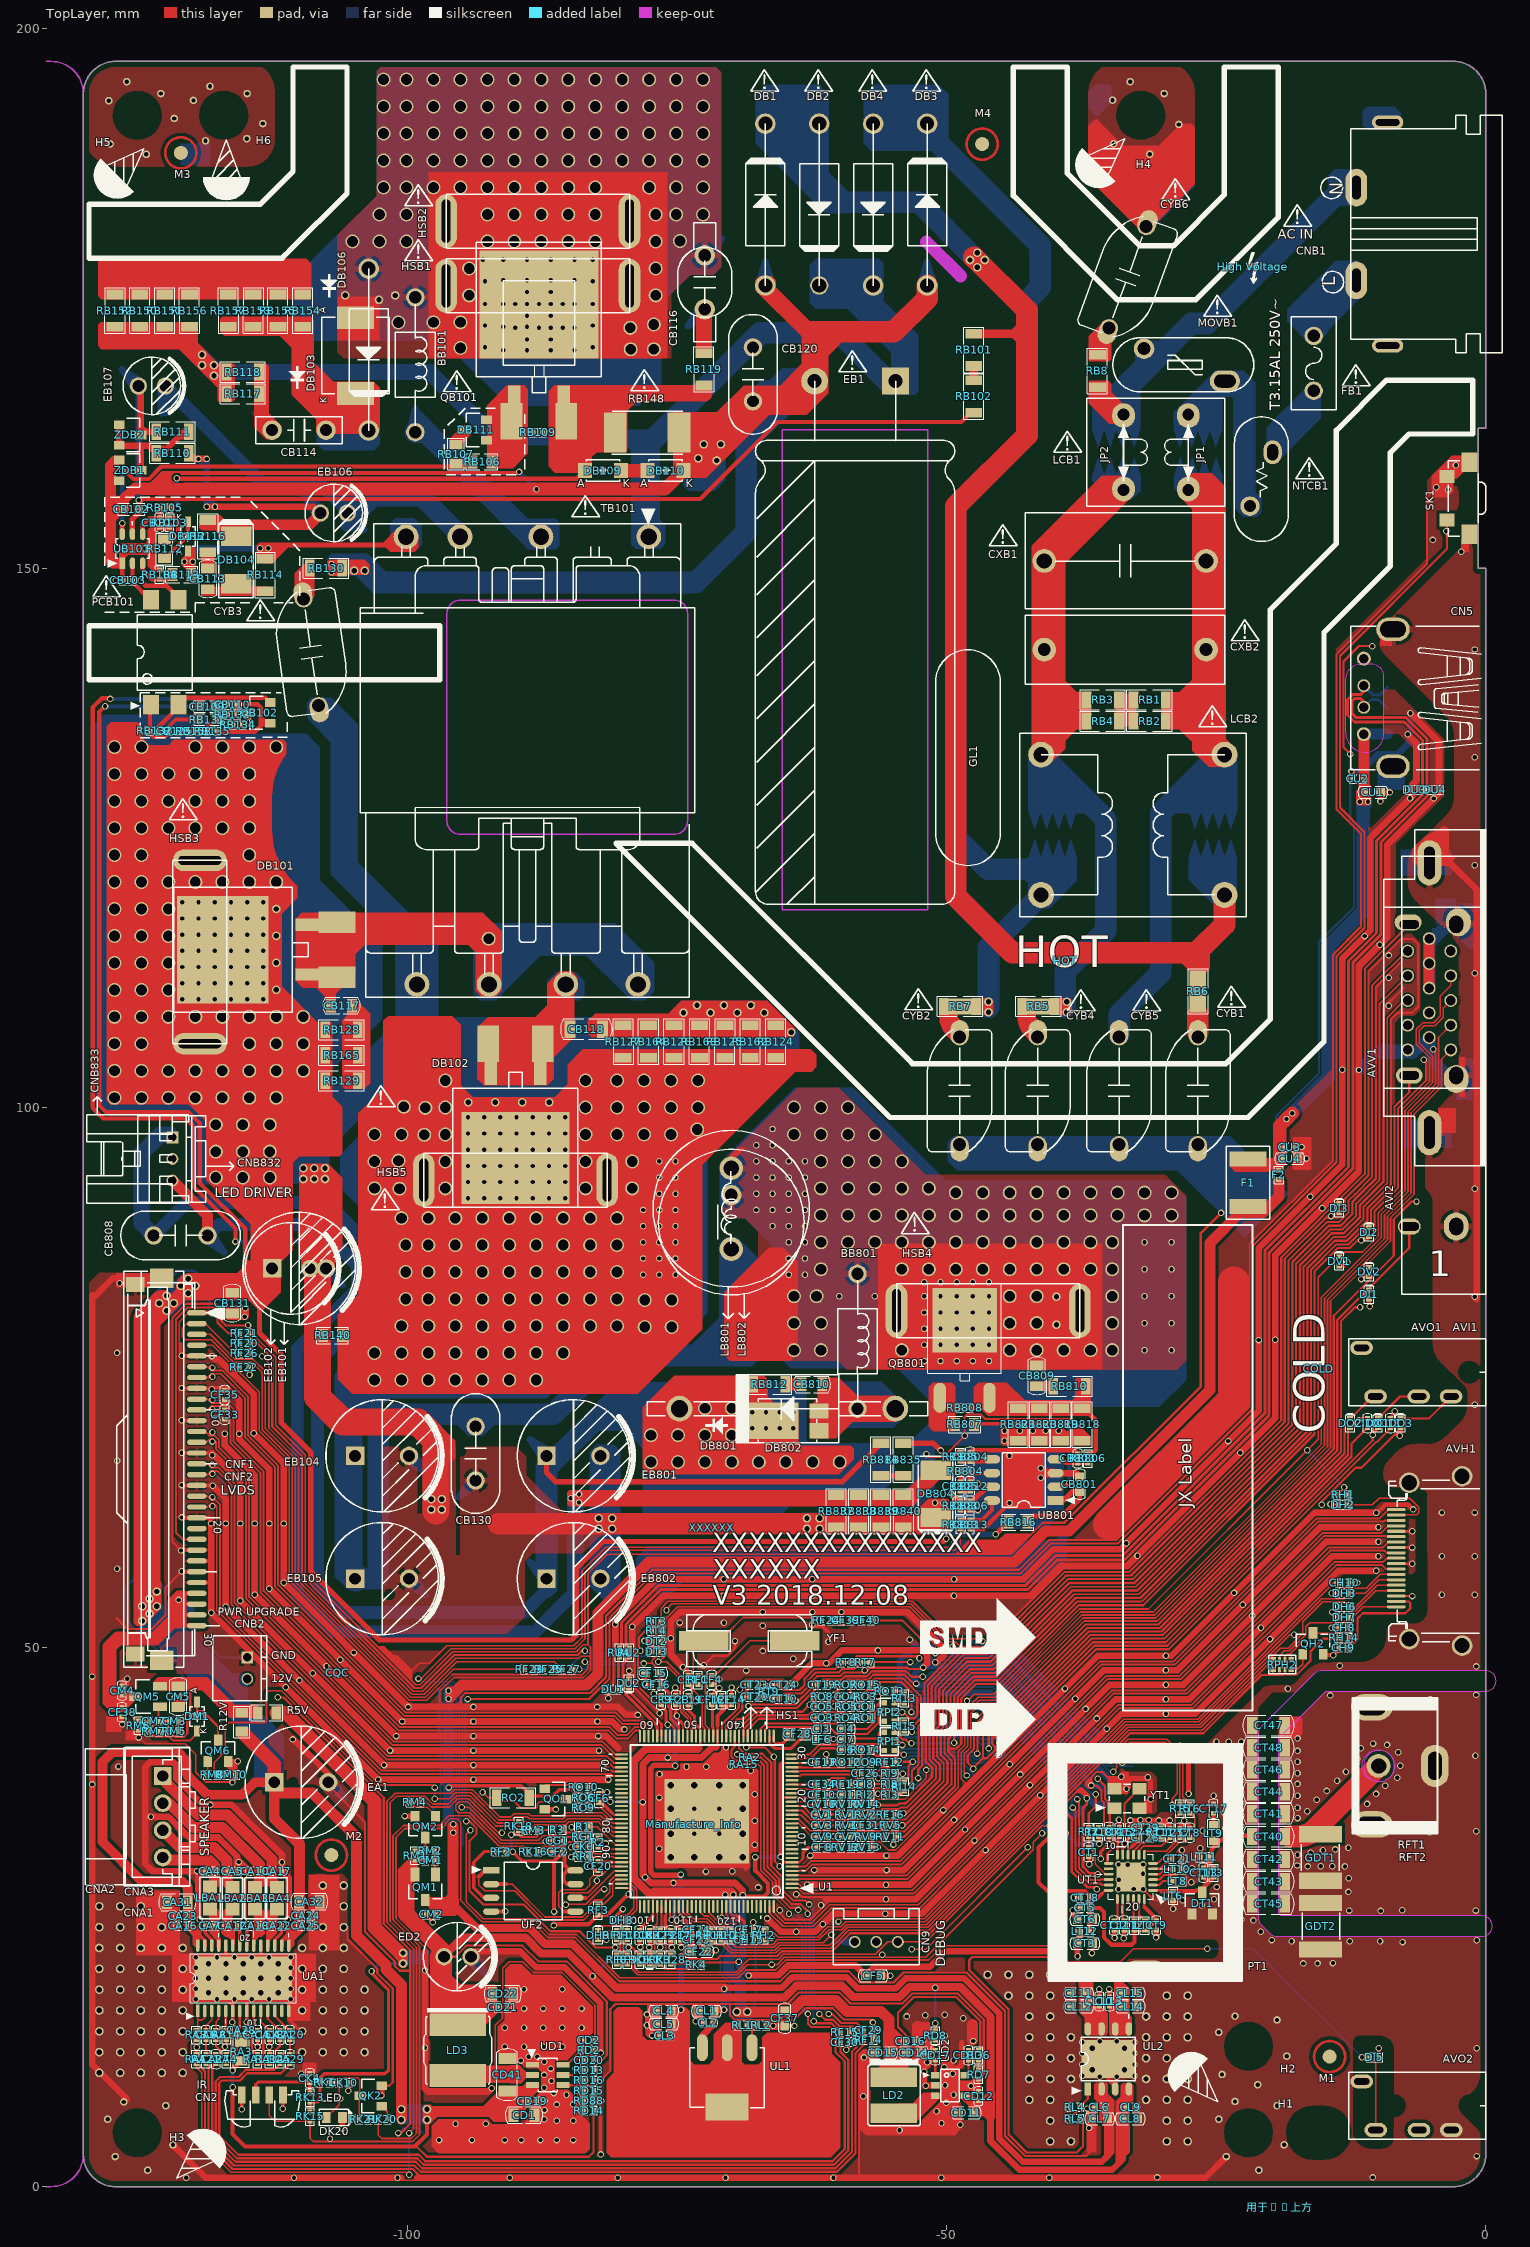
[diagram p0: TopLayer view]
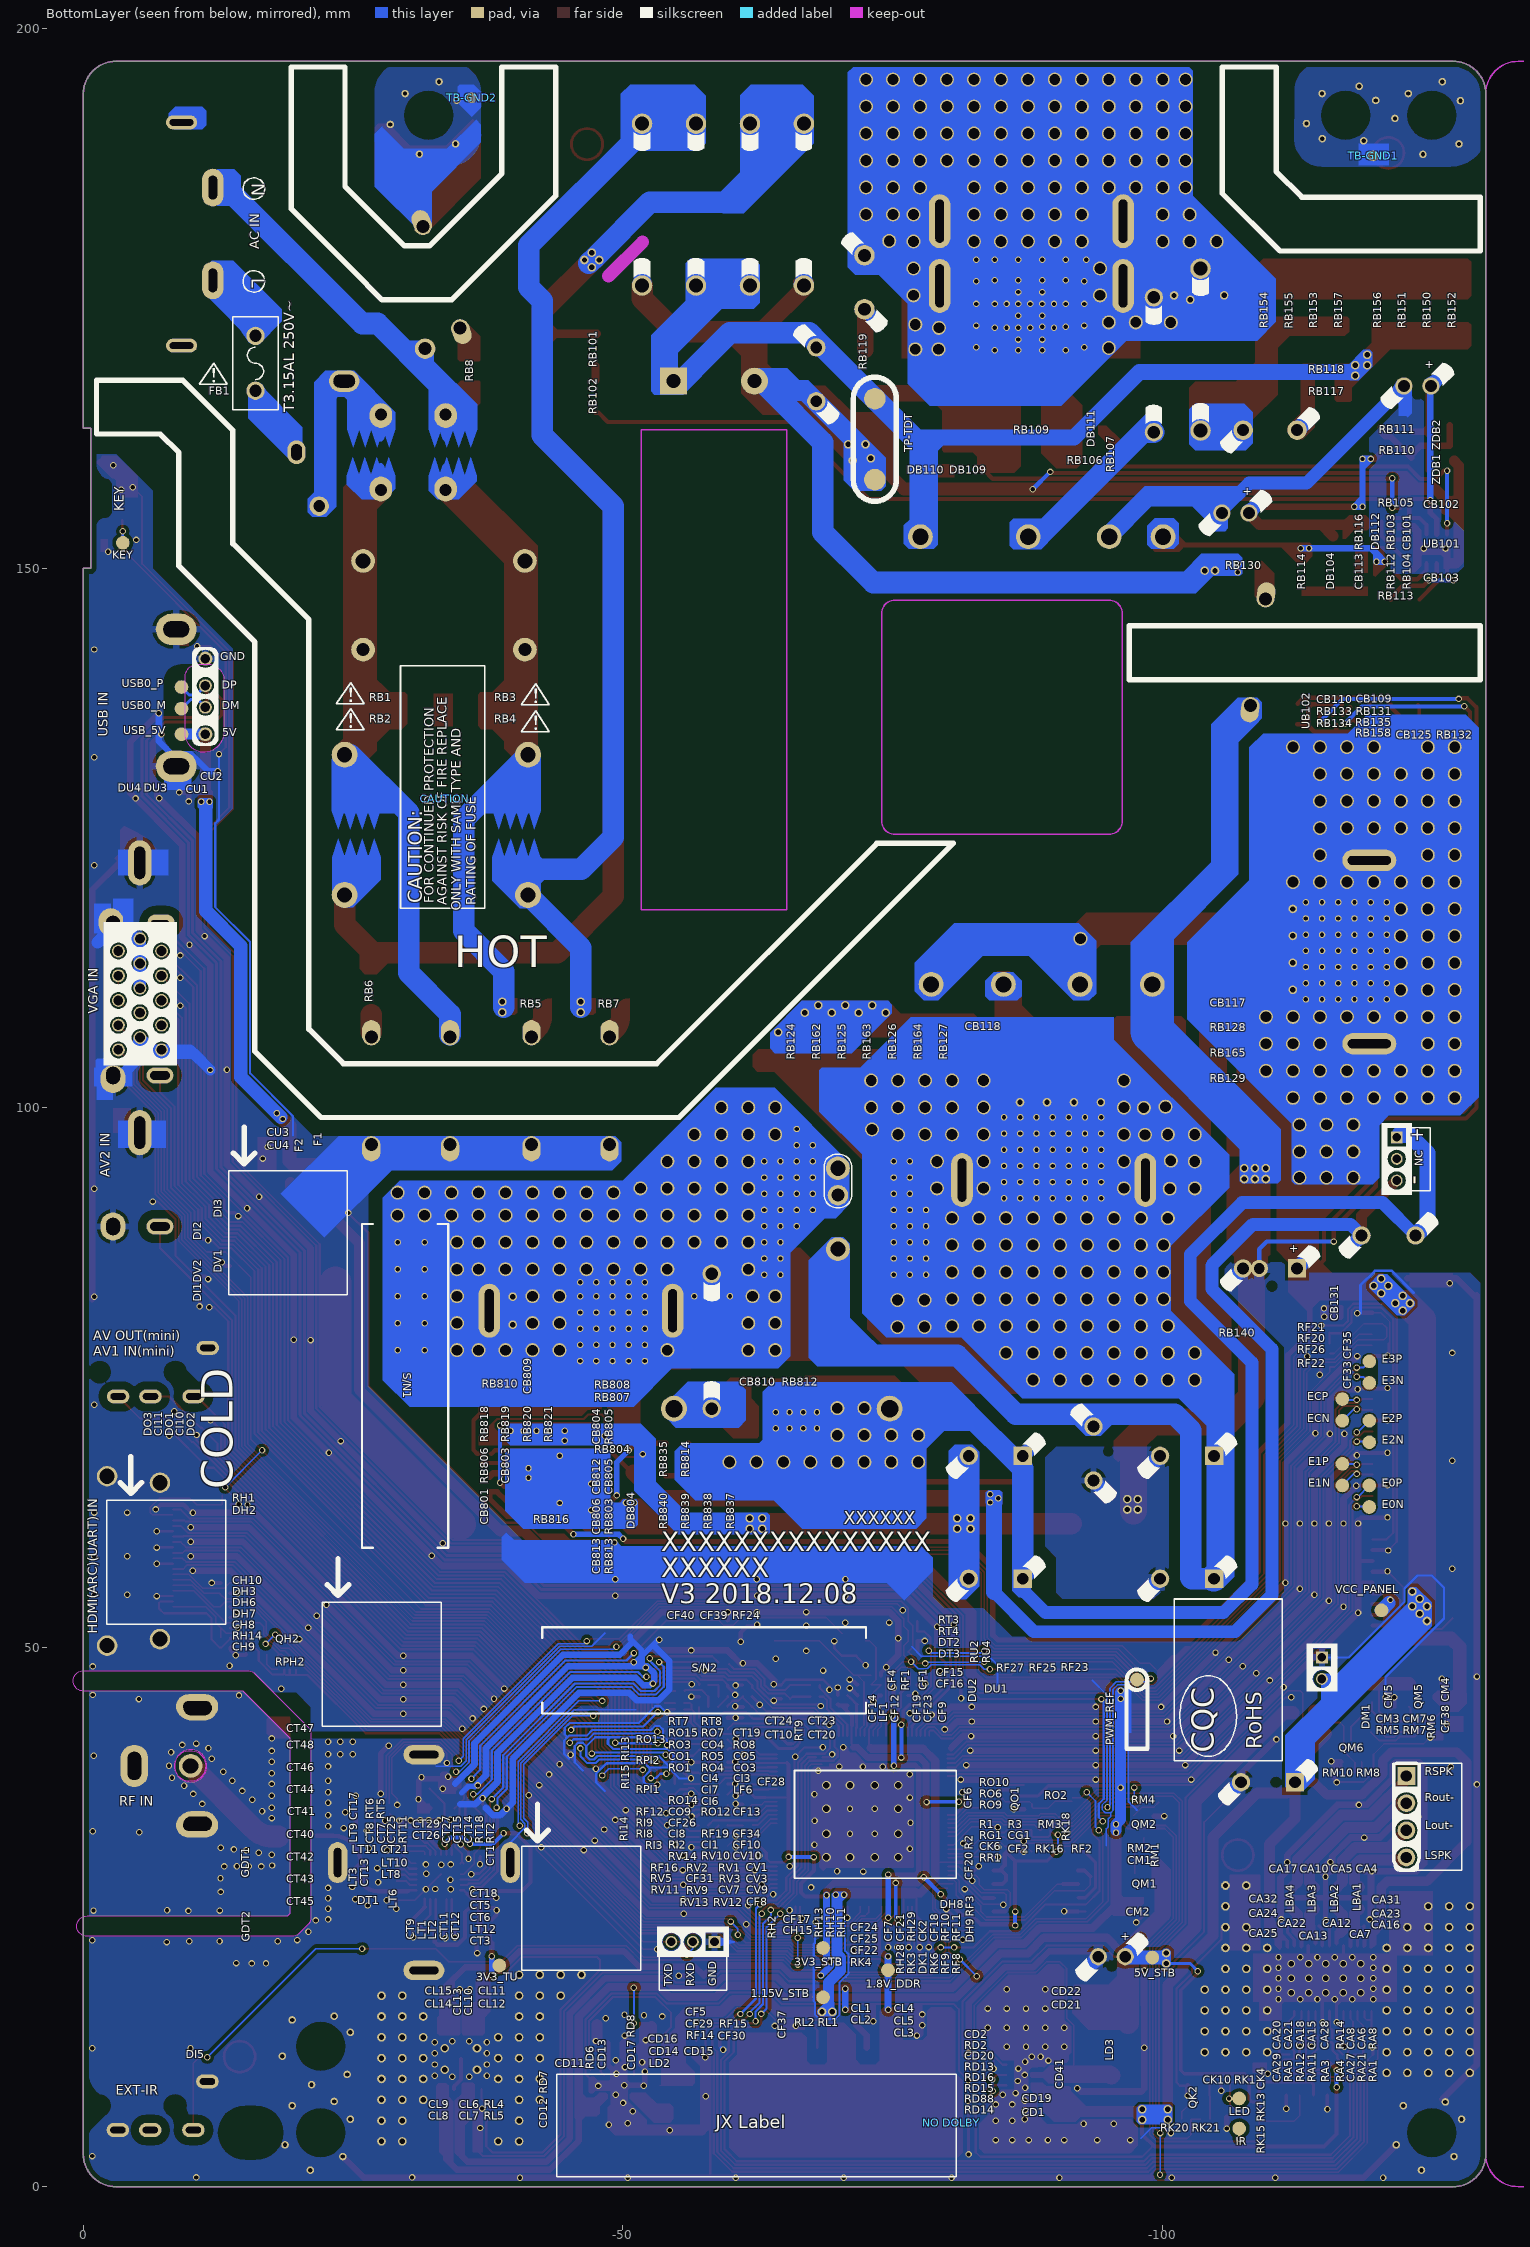
[diagram p1: BottomLayer view, seen from below]
# Altium PCB MISC84438.PcbDoc (part 1 of 15)
Units mm, origin at the board's own origin, x right, y up, seen from the top; angles counter-clockwise.
Board outline 130 x 197 mm, 2 copper layers (TopLayer, BottomLayer), stack 1.571 mm thick; 574 components, 314 nets, 2636 pads, 811 vias.

## Layer stack, top to bottom
TopLayer: signal copper 0.0356
Dielectric: core 1.5, FR-4, Dk 4.8
BottomLayer: signal copper 0.0356

## Board outline
-130,3 ccw(c-127,3) -127,0 -3,0 ccw(c-3,3) 0,3 0,150 -0.703,150 -0.703,163 0,163 0,194 ccw(c-3,194) -3,197 -127,197 ccw(c-127,194) -130,194

## Design rules (kind name [scope] priority, off if disabled: settings)
Clearance ■KEEPOUT_18mil [(IsTrack Or IsArc) And (AsMM(Width) < 1) And IsKeepOut vs Not IsPad] p1: gap=0.457
Clearance ■HOT_7.2mm [InNetClass('HOT') vs InNetClass('All Nets') And (Not InNetClass('HOT'))] p2: gap=7.2
Clearance ■DFM_NPTH_10mil [(IsPadHoleValid And (PadIsPlated=false) Or IsPad And ((AsMM(PadXSize_AllLayers) < 1) or (AsMM(PadYSize_AllLayers) < 1 )) And IsKeepout) OR HasFootprintPad('ASSE*','0') vs Not IsPad] p3: gap=0.254
Clearance ■DFM_20mil [(IsTrack or IsArc or IsPad) And IsKeepOut vs IsTrack or IsArc or InPoly] p4: gap=0.508
Clearance ■PWR_A12_8mil [(InNetClass('PWR_A12_8mil') or InNet('*12V*') or InNet('*24V*') or InNet('*PVCC*') or InNet('*19V*') or InNet('*AMP*POWER*') or InNet('*AMP*VCC*') or InNet('*LNB*')) and Not IsPad vs Not InPoly] p5: gap=0.203
Clearance ■PS_L2All_3.2mm [InNet('L-1') vs InNet('*')] p6: gap=3.2
Clearance ■PS_L2LN_1.5mm [InNet('L') Or InNet('L-2') Or InNet('L-3') Or InNet('L-4') Or InNet('L-5') Or InNet('L-6') vs InNet('L-N') And Not(InNet('L') Or InNet('L-2') Or InNet('L-3') Or InNet('L-4') Or InNet('L-5') Or InNet('L-6'))] p7: gap=1.5
Clearance ■PS_N2LN_1.5mm [InNet('N') OR InNet('N-1') OR InNet('N-2') OR InNet('N-3') OR InNet('N-4') OR InNet('N-5') OR InNet('N-6') vs InNet('L-N') And Not (InNet('N') OR InNet('N-1') OR InNet('N-2') OR InNet('N-3') OR InNet('N-4') OR InNet('N-5') OR InNet('N-6'))] p8: gap=1.5
Clearance ■PS_L2LN_3mm [InNet('L') Or InNet('L-2') Or InNet('L-3') Or InNet('L-4') Or InNet('L-5') Or InNet('L-6') vs InNet('*') And Not (InNet('L-N') Or InNet('L') Or InNet('L-2') Or InNet('L-3') Or InNet('L-4') Or InNet('L-5') Or InNet('L-6') Or OnLayer('KeepOutLayer'))] p9: gap=3
Clearance ■PS_N2LN_3mm [InNet('N') OR InNet('N-1') OR InNet('N-2') OR InNet('N-3') OR InNet('N-4') OR InNet('N-5') OR InNet('N-6') vs InNet('*') And Not (InNet('L-N') Or InNet('N') OR InNet('N-1') OR InNet('N-2') OR InNet('N-3') OR InNet('N-4') OR InNet('N-5') OR InNet('N-6') Or OnLayer('KeepOutLayer'))] p10: gap=3
Clearance ■SIP2GND_8mil [HasFootprint('SIP*') vs InPoly] p11: gap=0.203
Clearance ■Poly_4mil [InPolygonClass('Poly_4mil') vs Not InPoly] p12: gap=0.102
Clearance ■Poly_5mil [InPolygonClass('Poly_5mil') vs Not InPoly] p13: gap=0.127
Clearance ■Poly_6.2mil [InPolygonClass('Poly_6.2mil') vs Not InPoly] p14: gap=0.157
Clearance ■Poly_8mil [InPolygonClass('Poly_8mil') vs Not InPoly] p15: gap=0.203
Clearance ■ESD_10mil [HasFootprint('*IEC*') Or HasFootprint('*-F1*') Or HasFootprint('ANT-RF*')] p16: gap=0.254
Clearance ■ESD_20mil [HasFootprint('*SHIELD*')] p17: gap=0.508
Clearance ■C_RFGND_1.8mm [InNet('RFGND') vs Not (InNet('RF*IN*') OR InNet('NetCT28*'))] p18: gap=1.8
Clearance ■GND_12mil [InNet('GND') vs InPoly] p19: gap=0.305
Clearance ■ESD_30mil [(HasFootprint('SCART*') OR HasFootprint('AV*') OR HasFootprint('DB15*') OR HasFootprint('PHONE*')) vs OnBottomLayer] p20: gap=0.762
Clearance ■ESD_NT_30mil [HasFootprint('SCART*') Or HasFootprint('PHONE-HD-12') Or HasFootprint('PHONE-HD-17') Or HasFootprint('PHONE-HD-10') Or HasFootprint('PHONE-HD-26') vs InNet('GND') And OnTopLayer] p21: gap=0.762
Clearance ■DFM_TH_5mil [HasFootprint('GND') or HasFootprint('TP*') or HasFootprint('MARK*') or HasFootprint('SPARK_GAP') or HasFootprint('USB-HD-3-2') or HasFootprint('PHONE-HS-20') and Not IsRegion vs OnBottomlayer And IsPad OR IsPadHoleValid] p22: gap=0.127
Clearance ■DFM_HS60_5mil [InPadClass('HS60') vs InPadClass('HS60') OR IsPadHoleValid and not InPadClass('VIA5')] p23: gap=0.127
Clearance ■DFM_BCR_4mm [IsPadHoleValid vs IsBoardCutoutRegion] p24: gap=4
Clearance ■DFM_TH_4mm [OnBottomlayer And IsSMTPin vs IsPadHoleValid and not InPadClass('VIA5')] p25: gap=4
Clearance ■DFM_HS60_4mm [InPadClass('HS60') vs IsPad and OnBottomlayer] p26: gap=4
Clearance ■VIA2VIA_6.2mil [(IsVia OR InPadClass('VIA5')) And Not (IsVia And (AsMM(HoleDiameter) = 0.1)) vs (IsVia OR InPadClass('VIA5')) And Not (IsVia And (AsMM(HoleDiameter) = 0.1))] p27: gap=0.157
Clearance ■VIA2VIA_10.2mil [(IsVia OR InPadClass('VIA5')) And Not (IsVia And (AsMM(HoleDiameter) = 0.1)) vs (IsVia OR InPadClass('VIA5')) And Not (IsVia And (AsMM(HoleDiameter) = 0.1))] p28: gap=0.259
Clearance ■VIA2PAD_BGA_5mil [HasFootprint('BGA*') and IsPad vs (IsVia OR InPadClass('VIA5')) And Not (IsVia And (AsMM(HoleDiameter) = 0.1))] p29: gap=0.127
Clearance ■VIA2PAD_6mil [IsVia And Not (IsVia And (AsMM(HoleDiameter) = 0.1)) vs IsPad and Not HasFootprintPad('*','EPAD') and Not HasFootprintPad('*','257') and Not HasFootprintPad('TP','*') and Not HasFootprintPad  ('GND','JP*') and Not HasFootprintPad('LQFP216/0.4-2','217') and Not HasFootprintPad('QFP16*','17') and Not HasFootprintPad('QFN16*','17')  and Not HasFootprintPad('QFN20*','21') and Not HasFootprintPad('QFN24*','25') and Not HasFootprintPad( 'QFN24*','29') and Not  HasFootprintPad('QFN28*','29') and Not HasFootprintPad('QFN32*','33') and Not HasFootprintPad('QFN36*','37') and Not HasFootprintPad  ('QFN36*','0') and Not HasFootprintPad('QFN32*','0') and Not HasFootprintPad('QFN40*','41') and Not HasFootprintPad('QFN48*','49') and Not  HasFootprintPad('LQFP48/0.5-2','49') and Not HasFootprintPad('*SSOP32*','33') and Not HasFootprintPad('SOP8*','9') and Not HasFootprintPad  ('WSON8/1.27*','9') and Not HasFootprintPad('DFN10/0.5-1*','11') and Not HasFootprintPad('SON16/0.4','9') and Not HasFootprintPad  ('MSOP10/0.5-1','11') and Not HasFootprintPad('QFN56/0.5','57') and Not HasFootprintPad('LGA31/0.5','3*') and Not InPadClass('VIA_HS60')  and Not HasFootprintPad('TSSOP16/0.65-3','17') and Not HasFootprintPad('QFP128/0.5-2','129') and Not HasFootprintPad('QFP128/0.4-5','129')  and Not HasFootprintPad('PQFP48*','49') and Not HasFootprintPad('QFP156/0.4-1','157') and Not HasFootprintPad('D2PAK3','2')] p30: gap=0.152
Clearance ■PAD2VIA5_6mil [IsPad And ((AsMM(PadXSize_AllLayers) < 2.5) or ((AsMM(PadYSize_AllLayers) < 2.5))) And Not InPadclass('HS60') vs InPadClass('VIA5')] p31: gap=0.152
Clearance "■12mil for Polygon" [InPoly] p32: gap=0.305
Clearance 8mil [All] p33 off: gap=0.203
Clearance 7mil [All] p34 off: gap=0.178
Clearance 6.2mil [All] p35 off: gap=0.157
Clearance 6mil [All] p36 off: gap=0.152
Clearance 5.8mil [All] p37 off: gap=0.147
Clearance 5mil [Not ((IsTrack Or IsArc) And (Layer = 'KeepOutLayer')) vs Not (IsPad or ((IsTrack Or IsArc) And (Layer = 'KeepOutLayer')))] p38: gap=0.127
Clearance 4.5mil [Not ((IsTrack Or IsArc) And (Layer = 'KeepOutLayer')) vs Not (IsPad or ((IsTrack Or IsArc) And (Layer = 'KeepOutLayer')))] p39 off: gap=0.114
Clearance "4mil for Minimum" [Not ((IsTrack Or IsArc) And (Layer = 'KeepOutLayer')) vs Not (IsPad or ((IsTrack Or IsArc) And (Layer = 'KeepOutLayer')))] p40 off: gap=0.102
ComponentClearance [All] p1 off: gap=0.003 collisioncheckmode=3 verticalgap=1 showdistances=FALSE
DiffPairsRouting DiffPair_USB_DiffPairsRouting [InDifferentialPairClass('USB')] p1: maxlimit=0.127 minlimit=0.102 mostfreqgap=0.127 maxuncoupledlength=5.08
DiffPairsRouting DiffPair_LVDS_DiffPairsRouting [InDifferentialPairClass('LVDS')] p2: maxlimit=0.127 minlimit=0.102 mostfreqgap=0.127 maxuncoupledlength=12.7
DiffPairsRouting DiffPair_HDMI_DiffPairsRouting [InDifferentialPairClass('HDMI')] p3: maxlimit=0.127 minlimit=0.102 mostfreqgap=0.127 maxuncoupledlength=5.08
DiffPairsRouting [All] p4: maxlimit=0.254 minlimit=0.254 mostfreqgap=0.254 maxuncoupledlength=12.7
FabricationTestPointUsage TestPointUsage [All] p1: valid=0 allowmultiple=FALSE
FabricationTestpoint Testpoint [All] p1: side=3 testpointundercomponent=TRUE minsize=1.016 maxsize=2.54 preferedsize=1.524 minholesize=0.508 maxholesize=1.016 preferedholesize=0.813 testpointgrid=0.025 allowsidetop=TRUE allowsidebottom=TRUE usegrid=TRUE gridtolerance=0
HoleSize HoleSize_VIA [ISVIA] p1 off: absolutevalues=TRUE maxlimit=0.6 minlimit=0.2 maxpercent=80.000 minpercent=20.000
HoleToHoleClearance Hole2Hole [All] p1 off: gap=0.457 allowstackedmicrovias=FALSE
MatchedLengths DiffPair_USB_MatchedLengths [InDifferentialPairClass('USB')] p1: tolerance=2.54 checknetsindiffpair=TRUE checkdiffpairvsdiffpair=FALSE checkothers=FALSE
MatchedLengths DiffPair_LVDS_MatchedLengths [InDifferentialPairClass('LVDS')] p2: tolerance=2.54 checknetsindiffpair=TRUE checkdiffpairvsdiffpair=FALSE checkothers=FALSE
MatchedLengths DiffPair_HDMI_MatchedLengths [InDifferentialPairClass('HDMI')] p3: tolerance=2.54 checknetsindiffpair=TRUE checkdiffpairvsdiffpair=FALSE checkothers=FALSE
MinimumAnnularRing [All] p1: minimumring=0.1
MinimumSolderMaskSliver [All] p1 off: minsoldermaskwidth=-0.025
NetAntennae [Not (HasFootprint('ANT-7') or HasFootprint('ANT-BLUECORE'))] p1: netantennaetolerance=1.016
PermittedLayers [All] p1: toplayerpermitted=TRUE bottomlayerpermitted=TRUE
PlaneClearance Plane_ESD_30mil [(HasFootprint('SCART*') OR HasFootprint('AV*') OR HasFootprint('DB15*') OR HasFootprint('PHONE*'))] p1: clearance=0.762
PlaneClearance [All] p2: clearance=0.229
PlaneConnect Plane2Via [IsVia or InPadClass('VIA5')] p1: planeconnectstyle=Direct reliefexpansion=0.508 reliefentries=4 reliefconductorwidth=0.254 reliefairgap=0.254
PlaneConnect PlaneConnect_PAD [HasFootprint('ASSE*') OR InPadclass('HS60')] p2: planeconnectstyle=Direct reliefexpansion=0.508 reliefentries=4 reliefconductorwidth=0.254 reliefairgap=0.254
PlaneConnect [All] p3: planeconnectstyle=Relief reliefexpansion=0.305 reliefentries=4 reliefconductorwidth=0.762 reliefairgap=0.305
PolygonConnect PourOverVia [IsVia vs IsPolygon] p1: connectstyle=Direct reliefconductorwidth=0.254 reliefentries=4 polygonreliefangle="90 Angle"
PolygonConnect VIA5_HS60 [InPadclass('HS60') or InPadClass('VIA5') vs IsPolygon] p2: connectstyle=Direct reliefconductorwidth=0.254 reliefentries=4 polygonreliefangle="90 Angle"
PolygonConnect Polygon_RFGND [InNet('RFGND')] p3: connectstyle=Direct reliefconductorwidth=0.254 reliefentries=4 polygonreliefangle="90 Angle"
PolygonConnect ESD_SCART [HasFootprint('SCART*') vs IsPolygon And onBottomlayer] p4: connectstyle=Direct reliefconductorwidth=0.762 reliefentries=4 polygonreliefangle="90 Angle"
PolygonConnect FH2Polygon [HasFootprint('ASSE*') or HasFootprint('DIODE-S0402') or HasFootprint('RCL0524P') vs IsPolygon] p5: connectstyle=Direct reliefconductorwidth=0.254 reliefentries=4 polygonreliefangle="90 Angle"
PolygonConnect PWC1_2Polygon [(HasFootprint('*0805*') OR HasFootprint('*1206*')) vs IsPolygon] p6: connectstyle=Relief reliefconductorwidth=0.762 reliefentries=4 polygonreliefangle="90 Angle"
PolygonConnect PWC2_2Polygon [HasFootprint('*0603*') vs IsPolygon] p7: connectstyle=Relief reliefconductorwidth=0.635 reliefentries=4 polygonreliefangle="90 Angle"
PolygonConnect PWC3_2Polygon [HasFootprint('EC*') vs IsPolygon] p8: connectstyle=Relief reliefconductorwidth=0.889 reliefentries=4 polygonreliefangle="90 Angle"
PolygonConnect PWC2Polygon [(HasFootprint('SOT-89') OR HasFootprint('SOT-223') OR HasFootprint('TO-252') OR HasFootprint('TO-263') OR HasFootprint('DIODE') OR HasFootprint('SW-HS-2') OR HasFootprint('HDMI*') OR HasFootprint('SO-8B') OR HasFootprint('GND') OR HasFootprint('PHONE*') OR HasFootprint('DIP18/2.54-2') OR HasFootprint('DIP18/2.54-1') OR HasFootprint('UFL-R-SMT-1') OR HasFootprint('WIFI') OR HasFootprint('UM02BS') OR HasFootprint('*SCART*') OR HasFootprint('TSOT23-8/0.65') OR HasFootprint('*SOT-23-*') OR HasFootprint('SOP23-5-1') OR HasFootprint('SOP6/0.95') OR HasFootprint('M-WIFI-2-M603USA1') OR HasFootprint('M-MT7632U') OR HasFootprint('SOP8/1.27') OR HasFootprint('SOP8/1.27-3')) vs IsPolygon] p9: connectstyle=Direct reliefconductorwidth=0.889 reliefentries=4 polygonreliefangle="90 Angle"
PolygonConnect SMD2Polygon [IsSMTPin vs IsPolygon] p10: connectstyle=Relief reliefconductorwidth=0.305 reliefentries=4 polygonreliefangle="90 Angle"
PolygonConnect PTH2Polygon [IsThruPin vs IsPolygon] p11: connectstyle=Relief reliefconductorwidth=0.635 reliefentries=4 polygonreliefangle="90 Angle"
RoutingVias 0.6_0.4 [All] p1: holewidth=0.4 width=0.6 viastyle="Through Hole" minholewidth=0.4 minwidth=0.6 maxholewidth=0.4 maxwidth=0.6
RoutingVias 0.8_0.5 [All] p2 off: holewidth=0.5 width=0.8 viastyle="Through Hole" minholewidth=0.5 minwidth=0.8 maxholewidth=0.5 maxwidth=0.8
RoutingVias 0.5_0.3 [All] p3 off: holewidth=0.3 width=0.5 viastyle="Through Hole" minholewidth=0.3 minwidth=0.5 maxholewidth=0.3 maxwidth=0.5
RoutingVias 0.45_0.25 [All] p4 off: holewidth=0.25 width=0.45 viastyle="Through Hole" minholewidth=0.25 minwidth=0.45 maxholewidth=0.25 maxwidth=0.45
RoutingVias 0.4_0.2 [All] p5 off: holewidth=0.2 width=0.4 viastyle="Through Hole" minholewidth=0.2 minwidth=0.4 maxholewidth=0.2 maxwidth=0.4
RoutingVias 0.25_0.1 [All] p6 off: holewidth=0.1 width=0.25 viastyle="Through Hole" minholewidth=0.1 minwidth=0.25 maxholewidth=0.1 maxwidth=0.25
SMDNeckDown SMDNeckDown_Chip [HasFootprint('FFC*') or HasFootprint('QFP*') or HasFootprint('QFN*') or HasFootprint('HDMI*') or HasFootprint('BGA*')] p1: percent=100.000
SMDToCorner [All] p1 off: distance=40000
ShortCircuit ■ShortCircuit_ViaOnEpad [HasFootprintPad( '*','EPAD') vs IsVia AND InNet('*')] p1: allowed=TRUE
ShortCircuit ■ShortCircuit_JP [HasFootprintPad( 'GND','JP_1K') vs HasFootprintPad( 'GND','JP_2K')] p2: allowed=TRUE
ShortCircuit ■ShortCircuit_0402 [HasFootprintPad('R0402SC','1') Or HasFootprintPad('R0402SC','2') vs HasFootprintPad('R0402SC','3')] p3: allowed=TRUE
ShortCircuit ■ShortCircuit [InNet('*')] p4: allowed=FALSE
SilkToSilkClearance Silk2Silk [All] p1: silktosilkclearance=0.051
SilkscreenOverComponentPads [IsText] p1: minsilkscreentomaskgap=0.003
SolderMaskExpansion SolderMask_BGA [HasFootprint('BGA*') OR HasFootprint('*0201*')] p1: expansion=0.051
SolderMaskExpansion SolderMask_VIA [IsVia] p2: expansion=0.13
SolderMaskExpansion [All] p3: expansion=0.076
UnRoutedNet ■UnRoutedNet [All] p1:
ViasUnderSMD [All] p1: allowed=FALSE
Width DiffPair_USB_Width [InDifferentialPairClass('USB')] p1: maxlimit=0.279 minlimit=0.102 preferedwidth=0.279
Width DiffPair_LVDS_Width [InDifferentialPairClass('LVDS')] p2: maxlimit=0.178 minlimit=0.102 preferedwidth=0.178
Width DiffPair_HDMI_Width [InDifferentialPairClass('HDMI')] p3: maxlimit=0.178 minlimit=0.102 preferedwidth=0.178
Width [All] p4: maxlimit=6.35 minlimit=0.076 preferedwidth=0.203
14 further rules are at their usual default settings.

## Classes and differential pairs
polygon class Poly_6.2mil: 6.2
component class PCB_info: A13XX AI_V Barcode CAUTION COLD CQC DIP DOLBY H1 H2 H3 H4 H5 H6 "High Voltage" HOT M1 M2 M3 M4 Manufacture_Info S/N1 S/N2 SMD XXXXXXXXXXXXXXX
pad class VIA5: CF33-1 CF35-1 CL8-1 CL9-1 CL11-2 CL12-2 CL14-2 CL15-1 CT17-2 CT21-2 CT41-1 CT42-1 CT43-1 CT44-1 CT45-1 CT46-1 CT47-1 CT48-1 DT1-1 DT1-3 Free-VIA5 Free-via5 GDT2-1 LT6-2 LT8-2 LT11-2 PT1-1 PT1-2 PT1-3 PT1-4 RL4-1 UL2-3
pad class ShortCricuit_JP2: GND_JP1-JP_2K GND_JP2-JP_2K
pad class ShortCricuit_JP1: GND_JP1-JP_1K GND_JP2-JP_1K
pad class HS60: Free-HS60
differential pair class USB: DiffPair_USB_0
differential pair class HDMI: DiffPair_HDMI_0 DiffPair_HDMI_1 DiffPair_HDMI_2 DiffPair_HDMI_3
differential pair class LVDS: DiffPair_LVDS_0
polygon class Poly_5mil: 5
polygon class C_12mil: 12 GND
component class PS#01_XXXXXXXXXXXXXXX: BB101 BB102 BB801 CB101 CB102 CB103 CB109 CB110 CB113 CB114 CB116 CB117 CB118 CB120 CB125 CB130 CB131 CB801 CB803 CB804 CB805 CB806 CB808 CB809 CB810 CB812 CB813 CNB1 CNB2 CNB832 CNB833 "Conformal Coating" CXB1 CXB2 CYB1 CYB2 CYB3 CYB4 CYB5 CYB6 DB1 DB2 DB3 DB4 DB101 DB102 DB103 DB104 DB106 DB109 DB110 DB111 DB112 DB801 DB802 DB804 EB1 EB101 EB102 EB103 EB104 EB105 EB106 EB107 EB801 EB802 FB1 GL1 HSB1 HSB2 HSB3 HSB4 HSB5 HSB6 HSB7 JP1 JP2 LB801 LB802 LB803 LCB1 LCB2 LCB3 MOVB1 NTCB1 NTCB2 PCB101 PWM_REF QB101 QB801 RB1 RB2 RB3 RB4 RB5 RB6 RB7 RB8 RB101 RB102 RB103 RB104 RB105 RB106 RB107 RB109 RB110 RB111 RB112 RB113 RB114 RB115 RB116 RB117 RB118 RB119 RB124 RB125 RB126 RB127 RB128 RB129 RB130 RB131 RB132 RB133 RB134 RB135 RB140 RB148 RB150 RB151 RB152 RB153 RB154 RB155 RB156 RB157 RB158 RB162 RB163 RB164 RB165 RB803 RB804 RB805 RB806 RB807 RB808 RB810 RB812 RB813 RB814 RB816 RB818 RB819 RB820 RB821 RB835 RB837 RB838 RB839 RB840 TB101 TB-GND1 TB-GND2 TP-TDT UB101 UB102 UB801 ZDB1 ZDB2
component class SCH_info: HS1 "NO DOLBY" XXXXXX XXXXXXXXXXXXXXX 用于U1上方
component class TV#01_SYSTEM_POWER: 1.8V_DDR 1.15V_STB 3V3_STB 3V3_TU 5V_STB CD1 CD2 CD11 CD12 CD13 CD14 CD15 CD16 CD17 CD19 CD20 CD21 CD22 CD41 CG1 CL1 CL2 CL3 CL4 CL5 CL6 CL7 CL8 CL9 CL10 CL11 CL12 CL13 CL14 CL15 CM1 CM2 CM3 CM4 CM5 CM7 DM1 ED2 LD2 LD3 QM1 QM2 QM5 QM6 R5V R12V RD2 RD6 RD7 RD8 RD13 RD14 RD15 RD16 RD88 RG1 RL1 RL2 RL4 RL5 RM1 RM2 RM3 RM4 RM5 RM6 RM7 RM8 RM10 UD1 UD2 UL1 UL2 VCC_PANEL
component class TV#02_TSU69KR: CF1 CF2 CF4 CF5 CF6 CF7 CF8 CF9 CF10 CF12 CF13 CF14 CF15 CF16 CF17 CF18 CF19 CF20 CF21 CF22 CF23 CF24 CF25 CF26 CF28 CF29 CF30 CF31 CF34 CF37 CF39 CF40 LF1 LF6 R1 R2 R3 RF1 RF2 RF3 RF12 RF14 RF15 RF16 RF19 RF24 RR1 RT3 RT4 U1 UF2 YF1
component class TV#03_INTERFACE_INSIDE: CF33 CF35 CF38 CK2 CK4 CK6 CK10 CN2 CNF1 CNF2 DK1 DK20 E0N E0P E1N E1P E2N E2P E3N E3P ECN ECP IR KEY LED QK2 RF20 RF21 RF22 RF23 RF25 RF26 RF27 RK1 RK3 RK4 RK6 RK13 RK15 RK16 RK18 RK20 RK21 SK1
component class TV#04_INTERFACE_OUTSIDE: AVI1 AVI2 AVO1 AVO2 AVV1 CF31 CF34 CI1 CI3 CI4 CI6 CI7 CI8 CI10 CI11 CN5 CO1 CO3 CO4 CO5 CO9 CU1 CU2 CU3 CU4 CV1 CV3 CV7 CV9 CV10 DI1 DI2 DI3 DI5 DO1 DO2 DO3 DU1 DU2 DU3 DU4 DV1 DV2 F1 F2 QO1 RF16 RF19 RI2 RI3 RI8 RI9 RI13 RI14 RI15 RO1 RO2 RO3 RO4 RO5 RO6 RO7 RO8 RO9 RO10 RO12 RO13 RO14 RO15 RPI1 RPI2 RU2 RU4 RV1 RV2 RV3 RV5 RV9 RV10 RV11 RV12 RV13 RV14 USB0_M USB0_P USB_5V
component class TV#05_HDMI: AVH1 CH8 CH9 CH10 CH15 CN9 DH2 DH3 DH6 DH7 DH8 DH9 QH2 RF8 RF9 RF10 RF11 RH1 RH2 RH10 RH11 RH13 RH14 RH28 RH29 RPH2
component class TV#06_AMP_RDA3118E: CA4 CA5 CA6 CA7 CA8 CA10 CA12 CA13 CA15 CA16 CA17 CA18 CA20 CA21 CA22 CA23 CA24 CA25 CA27 CA28 CA29 CA31 CA32 CNA1 CNA2 CNA3 EA1 LBA1 LBA2 LBA3 LBA4 RA1 RA2 RA3 RA4 RA5 RA8 RA11 RA12 RA14 RA15 RA21 UA1
component class TV#07_TUNER_R842: CT1 CT3 CT5 CT6 CT7 CT8 CT9 CT10 CT11 CT12 CT13 CT14 CT15 CT17 CT18 CT19 CT20 CT21 CT23 CT24 CT25 CT26 CT27 CT29 CT40 CT41 CT42 CT43 CT44 CT45 CT46 CT47 CT48 DT1 DT2 DT3 GDT1 GDT2 LT1 LT2 LT3 LT6 LT8 LT9 LT10 LT11 LT12 PT1 RFT1 RFT2 RT2 RT5 RT6 RT7 RT8 RT9 RT11 RT18 UT1 YT1
net class HOT: 12V-OVP BRO D_QB101 L L-1 L-2 L-3 L-4 L-5 L-N N N-1 N-2 N-4 N-5 N-6 NetBB101_2 NetCB101_1 NetCB102_1 NetCB103_1 NetCB113_1 NetCB113_2 NetCB114_1 NetCB114_2 NetCB116_1 NetCNB1_3 NetCNB1_4 NetCYB3_1 NetCYB6_1 NetDB104_K NetDB109_A NetDB109_K NetDB111_1 NetDB111_2 NetDB112_K NetJP2_2 NetRB101_2 NetRB106_1 NetRB110_1 NetRB150_1 SGND Vbridge
net class POWER: 12V 12V-OVP BRO D_QB101 D_QB801 GND L L-1 L-2 L-3 L-4 L-5 L-N LED+ LED_CS LED_FB LED_GATE LED_OVP N N-1 N-2 N-4 N-5 N-6 NetBB101_2 NetBB801_2 NetCB101_1 NetCB102_1 NetCB103_1 NetCB109_1 NetCB109_2 NetCB110_2 NetCB113_1 NetCB113_2 NetCB114_1 NetCB114_2 NetCB116_1 NetCB117_1 NetCB117_2 NetCB118_1 NetCB118_2 NetCB125_1 NetCB125_2 NetCB801_2 NetCB803_1 NetCB804_1 NetCB805_2 NetCB809_1 NetCB810_2 NetCB812_2 NetCB813_2 NetCNB1_3 NetCNB1_4 NetCNB832_2 NetCYB3_1 NetCYB6_1 NetDB104_K NetDB109_A NetDB109_K NetDB111_1 NetDB111_2 NetDB112_K NetJP2_2 NetQB801_G NetRB101_2 NetRB106_1 NetRB110_1 NetRB150_1 NetRB814_2 PWM_REF SGND VBL Vbridge
net class HDMI_Net: HDMI1_RX0_N HDMI1_RX0_P HDMI1_RX1_N HDMI1_RX1_P HDMI1_RX2_N HDMI1_RX2_P HDMI1_RXC_N HDMI1_RXC_P USB0_M USB0_P
net class USB_Net: USB0_M USB0_P
net class LVDS_Net: RXE3+ RXE3-
differential pair DiffPair_USB_0: +USB0_M -USB0_P
differential pair DiffPair_HDMI_0: +HDMI1_RX2_N -HDMI1_RX2_P
differential pair DiffPair_HDMI_1: +HDMI1_RX1_N -HDMI1_RX1_P
differential pair DiffPair_HDMI_2: +HDMI1_RX0_N -HDMI1_RX0_P
differential pair DiffPair_HDMI_3: +HDMI1_RXC_N -HDMI1_RXC_P
differential pair DiffPair_LVDS_0: +RXE3+ -RXE3-

## Components (designator, comment, footprint, x,y, rotation, side; value= is the part's Value field where it differs from the comment)
1.8V_DDR "TEST" TP -74.587,20.066 r180 bottom
1.15V_STB "TEST" TP -68.567,17.551 r270 bottom
3V3_STB "TEST" TP -68.567,22.123 r90 bottom
3V3_TU "TEST" TP -38.557,20.498 r270 bottom
5V_STB "TEST" TP -99.085,21.234 r0 bottom
AI_V "AI_GRIPPER_V" AI_GRIPPER_V 256.019,35.242 r90 top
AVH1 "HDMI terminal,HDMI Jack,H,Block up,SMD,51U019S-313HFN-E-R-F,FREEPORT" HDMI-HS-11 -0.6,58 r90 top locked
AVI1 "NC/Earphone terminal,Earphone Jack,H,Φ3.6,CH5.5,Black,Seal,DIP,PJ-320B-Φ5.5,JSL" PHONE-HD-43 -0.022,75.5 r90 top locked
AVI2 "RCA terminal,RCA Jack,AV3,H,Red, White, Yellow,CH5.5,D14,Seal,DIP,RC075-F03L3BY-L,YUQIU" AV3-H14-15 0,103 r90 top locked
AVO1 "Earphone terminal,Earphone Jack,H,Φ3.6,CH5.5,Black,Seal,DIP,PJ-320B-Φ5.5,JSL" PHONE-HD-43 -0.022,75.5 r90 top locked
AVO2 "NC/Earphone terminal,Earphone Jack,H,Φ3.6,CH5.5,Black,Seal,DIP,PJ-320B-Φ5.5,JSL" PHONE-HD-43 0,7.5 r90 top locked
AVV1 "NC/WLHD-051A" DB15-HF-1 0,110.2 r90 top locked
BB101 "Ferrite bead,BEAD,70ohmMin,φ3.5×6.0×0.65,DIP,TP,RH3.5×6×0.8-T-LF,DL" LB/3.5*6*12.5#1 -99.228,168.873 r270 top
BB801 "Ferrite bead,BEAD,30ohmMin,Φ3.5×3.0×0.65,DIP,TP,RH3.5×3×0.8-T-LF,DL" LB/3.5*6*12.5#2 -58.242,78.364 r270 top
CA4 "2200pF-0402-X7R-±10%-50V" C0402 -118.274,29.248 r180 top
CA5 "2200pF-0402-X7R-±10%-50V" C0402 -116.191,29.248 r0 top
CA6 "0.22uF-0402-X5R-±10%-16V" C0402 -118.629,14.057 r270 top
CA7 "0.22uF-0402-X5R-±10%-16V" C0402 -118.274,24.179 r0 top
CA8 "0.22uF-0402-X5R-±10%-16V" C0402 -117.715,14.057 r270 top
CA10 "2200pF-0402-X7R-±10%-50V" C0402 -114.108,29.248 r180 top
CA12 "0.22uF-0402-X5R-±10%-16V" C0402 -116.191,24.178 r180 top
CA13 "0.22uF-0402-X5R-±10%-16V" C0402 -114.108,24.179 r0 top
CA15 "0.1uF-0402-X5R-±20%-16V" C0402 -113.854,14.057 r270 top
CA16 "NC/1000pF-0402-X7R-±10%-50V" C0402 -120.791,24.161 r0 top
CA17 "2200pF-0402-X7R-±10%-50V" C0402 -112.051,29.248 r180 top
CA18 "1uF-0402-X5R-±20%-16V" C0402 -112.737,14.057 r270 top
CA20 "0.22uF-0402-X5R-±10%-16V" C0402 -110.857,14.057 r270 top
CA21 "0.22uF-0402-X5R-±10%-16V" C0402 -111.771,14.057 r270 top
CA22 "0.22uF-0402-X5R-±10%-16V" C0402 -112.051,24.178 r180 top
CA23 "NC/0.1uF-0402-X5R-±20%-16V" C0402 -120.791,25.063 r0 top
CA24 "0.1uF-0402-X5R-±20%-16V" C0402 -109.383,25.102 r180 top
CA25 "NC/1000pF-0402-X7R-±10%-50V" C0402 -109.383,24.187 r180 top
CA27 "3300pF-0402-X7R-±10%-50V" C0402 -117.715,11.822 r270 top
CA28 "1uF-0402-X5R-±20%-16V" C0402 -115.341,14.503 r180 top
CA29 "3300pF-0402-X7R-±10%-50V" C0402 -110.857,11.822 r270 top
CA31 "10uF-0805-X5R-±20%-16V" C0805 -121.285,26.365 r0 top
CA32 "NC/10uF-0805-X5R-±20%-16V" C0805 -109.054,26.429 r180 top
CAUTION "CAUTION" CAUTION -33.477,128.651 r90 bottom
CB101 "100pF-0402-NPO-±5%-50V" C0402 -122.936,154.254 r270 top
CB102 "0.1uF-0603-X7R-±10%-50V" C0603 -125.565,155.473 r180 top
CB103 "Ceramic capacitor,CAP MC,50V,1000pF,±20%,X7R,0402,SMD,TP" C0402 -125.882,148.882 r180 top
CB109 "Ceramic capacitor,CAP MC,25V,0.22uF,±10%,X7R,0603,SMD,TP" C0603 -118.504,137.198 r0 top
CB110 "NC/1000pF-0402-X7R-±10%-50V" C0402 -116.205,137.35 r0 top
CB113 "NC/220PF-0805-NPO-±10%-200V" C0805 -118.478,149.022 r90 top
CB114 "Film capacitor,CAP PE,400V,4700pF,±5%,P,5.0mm,PC,DIP,TP,Fara" CAP8*2.5-V-5 -110.007,162.814 r0 top locked
CB116 "Ceramic capacitor,CAP CD,2KV,68pF,±5%,SL,IK,5.0mm,DIP,TP,Walsin" CAP6.5*5-V-5-1 -72.401,176.521 r90 top locked
CB117 "1000pF-0805-NPO-±10%-200V" C0805 -106.07,109.479 r0 top
CB118 "Ceramic capacitor,CAP MC,1KV,1000pF,±5%,NPO,1206,SMD,TP" C1206 -83.384,107.288 r0 top
CB120 "Ceramic capacitor,CAP CD,2KV,4700pF,±20%,Y5U,IK,5.0mm,DIP,TP,Walsin" CAP10*4.5-V-5#1 -67.939,167.989 r90 top
CB125 "NC/Ceramic capacitor,CAP MC,50V,0.022uF,±10%,X7R,0402,SMD,TP" C0402 -121.59,134.925 r0 top
CB130 "Ceramic capacitor,CAP CD,1KV,4700pF,±20%,Y5U,IK,5.0mm,DIP,TP,Walsin" CAP10*4.5-V-5#2 -93.638,67.958 r90 top locked
CB131 "Ceramic capacitor,CAP MC,200V,100pF,±5%,NPO,0805,SMD,TP" C0805 -116.2,81.9 r270 top
CB801 "Ceramic capacitor,CAP MC,25V,1uF,±10%,X7R,0603,SMD,TP" C0603 -37.668,65.113 r270 top
CB803 "100pF-0402-NPO-±5%-50V" C0402 -37.821,67.496 r90 top
CB804 "4700pF-0402-X7R-±10%-50V" C0402 -47.803,67.653 r90 top
CB805 "NC/0.1uF-0402-X7R-±10%-16V" C0402 -48.73,64.91 r90 top
CB806 "Ceramic capacitor,CAP MC,50V,1000pF,±20%,X7R,0402,SMD,TP" C0402 -47.803,63.132 r270 top
CB808 "NC/Ceramic capacitor,CAP CD,1KV,4700pF,±20%,Y5U,K,5.0mm,DIP,TP,Walsin" CAP10*4.5-V-5#3 -120.983,88.168 r180 top
CB809 "Ceramic capacitor,CAP MC,500V,220pF,±5%,NPO,0805,SMD,TP" C0805 -41.618,75.146 r90 top
CB810 "Ceramic capacitor,CAP MC,500V,220pF,±5%,NPO,0805,SMD,TP" C0805 -62.466,74.364 r180 top
CB812 "0.033uF-0402-X7R-±10%-16V" C0402 -47.803,64.91 r90 top